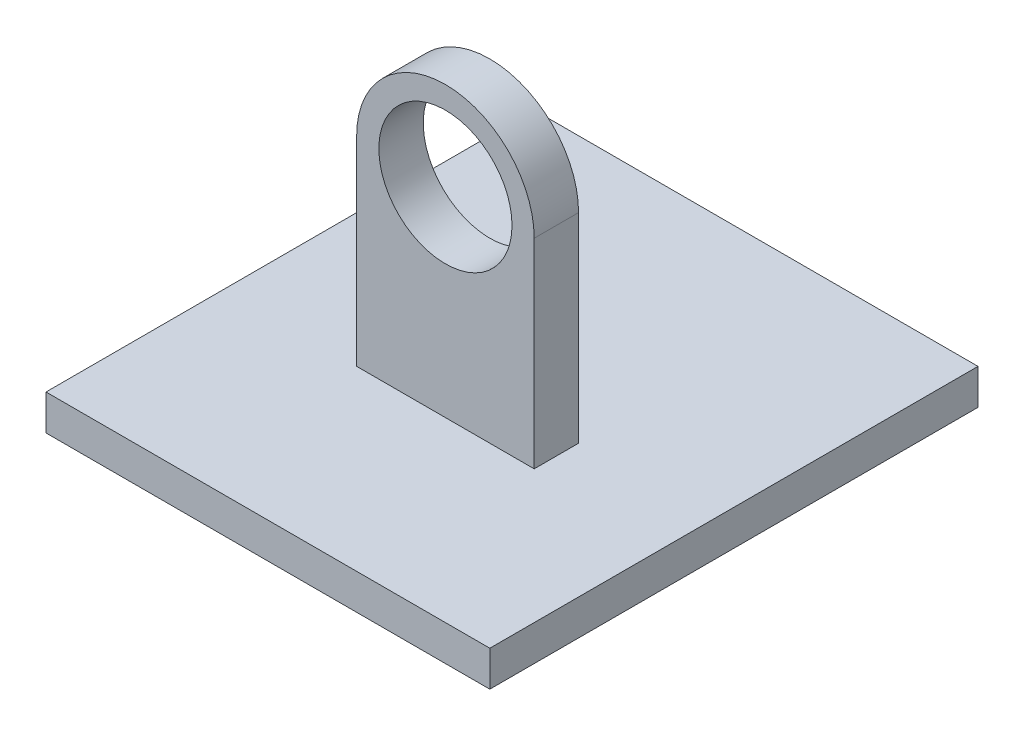
from build123d import *

# Parameters (mm, degrees)
SKETCH1_R           = 15
BOSS_EXTRUDE1_DEPTH = 10
SKETCH2_W           = 100
SKETCH2_H           = 110
BOSS_EXTRUDE2_DEPTH = 10
CHAMFER1_SIZE       = 2


with BuildPart() as part:
    # Sketch1 → Boss-Extrude1 (new body)
    with BuildSketch(Plane.XY):
        with BuildLine():
            Line((139, -40), (139, -85))
            Line((139, -85), (99, -85))
            Line((99, -85), (99, -40))
            ThreePointArc((99, -40), (119, -20), (139, -40))
        make_face()
        with Locations((119, -40)):
            Circle(SKETCH1_R, mode=Mode.SUBTRACT)
    extrude(amount=-BOSS_EXTRUDE1_DEPTH)

    # Sketch2 → Boss-Extrude2 (add)
    with BuildSketch(Plane.XZ.offset(85)):
        with Locations((119, -15)):
            Rectangle(SKETCH2_W, SKETCH2_H)
    extrude(amount=BOSS_EXTRUDE2_DEPTH)

    # Chamfer1
    chamfer1_edges = [part.edges().sort_by_distance(p)[0] for p in [
        (169, -95, -15),
        (119, -95, 40),
        (69, -95, -15),
        (119, -95, -70),
    ]]
    chamfer(chamfer1_edges, length=CHAMFER1_SIZE)


solid = part.part
